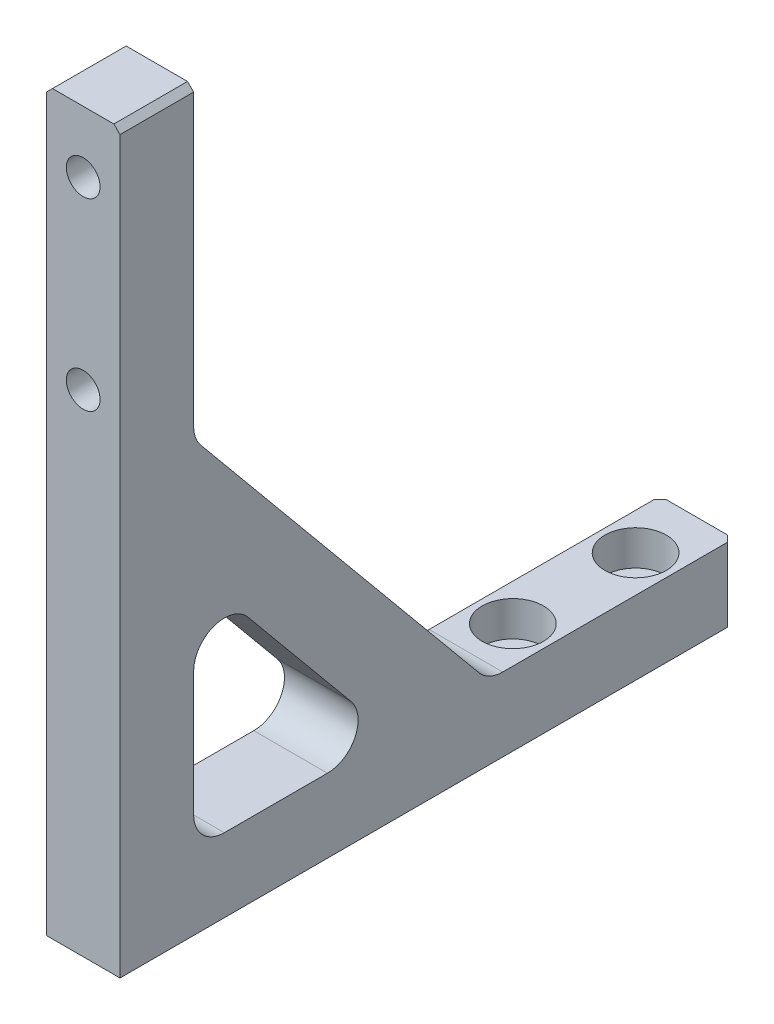
from build123d import *

# Parameters (mm, degrees)
BOSS_EXTRUDE1_DEPTH                                  = 12
CUT_EXTRUDE1_DEPTH                                   = 157.665248221
CBORE_FOR_M5_HEXAGON_SOCKET_HEAD_CAP_SCR_D           = 5.5
CBORE_FOR_M5_HEXAGON_SOCKET_HEAD_CAP_SCR_CBORE_D     = 10
CBORE_FOR_M5_HEXAGON_SOCKET_HEAD_CAP_SCR_CBORE_DEPTH = 5.7
CBORE_FOR_M5_HEXAGON_SOCKET_HEAD_CAP_2_D             = 5.5
CBORE_FOR_M5_HEXAGON_SOCKET_HEAD_CAP_2_CBORE_D       = 10
CBORE_FOR_M5_HEXAGON_SOCKET_HEAD_CAP_2_CBORE_DEPTH   = 5.7
CHAMFER1_SIZE                                        = 1
FILLET1_R                                            = 5


with BuildPart() as part:
    # Sketch1 → Boss-Extrude1 (new body)
    with BuildSketch(Plane(origin=(0, 0, 0), x_dir=(0, 0, -1), z_dir=(1, 0, 0))):
        Polygon((0, 0), (0, 120), (12, 120), (12, 70), (60, 12), (100, 12), (100, 0), align=None)
    extrude(amount=BOSS_EXTRUDE1_DEPTH)

    # Sketch2 → Cut-Extrude1 (cut, through all)
    with BuildSketch(Plane(origin=(12, 0, 0), x_dir=(0, 0, -1), z_dir=(1, 0, 0))):
        with BuildLine():
            Line((12, 37.294498848), (12, 17))
            ThreePointArc((12, 17), (13.464466094, 13.464466094), (17, 12))
            Line((17, 12), (33.795447323, 12))
            ThreePointArc((33.795447323, 12), (38.319781133, 14.871525529), (37.647418928, 20.18783857))
            Line((37.647418928, 20.18783857), (20.851971606, 40.482337418))
            ThreePointArc((20.851971606, 40.482337418), (15.305871615, 41.998744698), (12, 37.294498848))
        make_face()
    extrude(amount=-CUT_EXTRUDE1_DEPTH, mode=Mode.SUBTRACT)

    # CBORE for M5 Hexagon socket head cap scr (through all)
    with Locations(Plane(origin=(0, 0, -12), x_dir=(-1, 0, 0), z_dir=(0, 0, -1))):
        with Locations((-6, 80), (-6, 110)):
            CounterBoreHole(CBORE_FOR_M5_HEXAGON_SOCKET_HEAD_CAP_SCR_D / 2, CBORE_FOR_M5_HEXAGON_SOCKET_HEAD_CAP_SCR_CBORE_D / 2, CBORE_FOR_M5_HEXAGON_SOCKET_HEAD_CAP_SCR_CBORE_DEPTH)

    # CBORE for M5 Hexagon socket head cap 2 (through all)
    with Locations(Plane(origin=(0, 12, 0), x_dir=(1, 0, 0), z_dir=(0, 1, 0))):
        with Locations((6, 70), (6, 90)):
            CounterBoreHole(CBORE_FOR_M5_HEXAGON_SOCKET_HEAD_CAP_2_D / 2, CBORE_FOR_M5_HEXAGON_SOCKET_HEAD_CAP_2_CBORE_D / 2, CBORE_FOR_M5_HEXAGON_SOCKET_HEAD_CAP_2_CBORE_DEPTH)

    # Chamfer1
    chamfer1_edges = [part.edges().sort_by_distance(p)[0] for p in [
        (12, 120, -6),
        (0, 120, -6),
        (12, 6, -100),
        (0, 6, -100),
    ]]
    chamfer(chamfer1_edges, length=CHAMFER1_SIZE)

    # Fillet1
    fillet1_edges = [part.edges().sort_by_distance(p)[0] for p in [
        (6, 70, -12),
        (6, 12, -60),
    ]]
    fillet(fillet1_edges, radius=FILLET1_R)


solid = part.part
